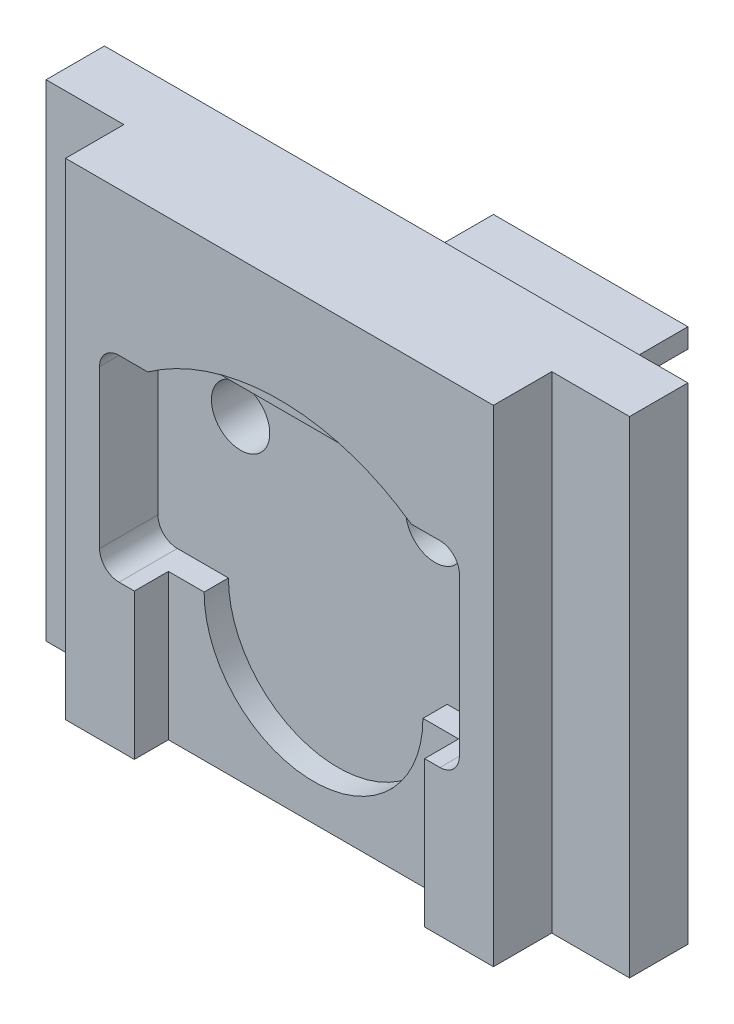
SolidWorks part; units mm, degrees
material "45"
ref_plane "前视基准面" through (0, 0, 0) normal (0, 0, 1) x (1, 0, 0)
ref_plane "上视基准面" through (0, 0, 0) normal (0, 1, 0) x (1, 0, 0)
ref_plane "右视基准面" through (0, 0, 0) normal (1, 0, 0) x (0, 0, -1)
sketch "草图1" plane through (0, 0, 0) normal (0, 0, 1) x (1, 0, 0)
  line L1 (30, -25) -> (-30, -25)
  line L2 (30, -25) -> (30, 25)
  line L3 (30, 25) -> (-30, 25)
  line L4 (-30, -25) -> (-30, 25)
  line L5 (30, -25) -> (-30, 25) construction
  line L6 (30, 25) -> (-30, -25) construction
  point P0 (0, 0)
  dimension "D1" = 60
  dimension "D2" = 50
extrude "凸台-拉伸1" add sketch "草图1" along normal blind 12
sketch "草图2" plane through (0, 0, 0) normal (0, 0, -1) x (-1, 0, 0)
  line L1 (10, -10) -> (-10, -10)
  line L2 (10, -10) -> (10, 10)
  line L3 (10, 10) -> (-10, 10)
  line L4 (-10, -10) -> (-10, 10)
  line L5 (10, -10) -> (-10, 10) construction
  line L6 (10, 10) -> (-10, -10) construction
  point P0 (0, 0)
  dimension "D1" = 20
  dimension "D2" = 20
extrude "凸台-拉伸2" add sketch "草图2" along normal blind 20
sketch "草图3" plane through (0, 0, 12) normal (0, 0, 1) x (1, 0, 0)
  line L0 (0, -25) -> (0, -10) construction
  line L1 (-30, -25) -> (30, -25) construction
  circle A0 centre (0, -10) radius 10.5
  dimension "D1" = 21
  dimension "D2" = 15
extrude "切除-拉伸1" cut sketch "草图3" against normal blind 6
sketch "草图5" plane through (0, 0, 12) normal (0, 0, 1) x (1, 0, 0)
  line L8 (-18.5, 4.9642) -> (-18.5, -1.5)
  line L9 (-17, -3) -> (-12.8452, -3)
  line L10 (12.8452, -3) -> (17, -3)
  line L11 (18.5, -1.5) -> (18.5, 4.9642)
  line L12 (-18.5, 4.9642) -> (-18.5, -1.5)
  line L13 (-17, -3) -> (-12.8452, -3)
  line L14 (12.8452, -3) -> (17, -3)
  line L15 (18.5, -1.5) -> (18.5, 4.9642)
  arc A16 (18.5, 4.9642) -> (18.1591, 5.9163) centre (17, 4.9642) ccw
  arc A17 (18.1591, 5.9163) -> (-18.1591, 5.9163) centre (0, -9) ccw
  arc A18 (-18.1591, 5.9163) -> (-18.5, 4.9642) centre (-17, 4.9642) ccw
  arc A19 (-18.5, -1.5) -> (-17, -3) centre (-17, -1.5) ccw
  arc A20 (-12.8452, -3) -> (-11.8311, -2.6053) centre (-12.8452, -1.5) ccw
  arc A21 (11.8311, -2.6053) -> (-11.8311, -2.6053) centre (0, -15.5) ccw
  arc A22 (11.8311, -2.6053) -> (12.8452, -3) centre (12.8452, -1.5) ccw
  arc A23 (17, -3) -> (18.5, -1.5) centre (17, -1.5) ccw
  arc A24 (18.5, 4.9642) -> (18.1591, 5.9163) centre (17, 4.9642) ccw
  arc A25 (18.1591, 5.9163) -> (-18.1591, 5.9163) centre (0, -9) ccw
  arc A26 (-18.1591, 5.9163) -> (-18.5, 4.9642) centre (-17, 4.9642) ccw
  arc A27 (-18.5, -1.5) -> (-17, -3) centre (-17, -1.5) ccw
  arc A28 (-12.8452, -3) -> (-11.8311, -2.6053) centre (-12.8452, -1.5) ccw
  arc A29 (11.8311, -2.6053) -> (-11.8311, -2.6053) centre (0, -15.5) ccw
  arc A30 (11.8311, -2.6053) -> (12.8452, -3) centre (12.8452, -1.5) ccw
  arc A31 (17, -3) -> (18.5, -1.5) centre (17, -1.5) ccw
  dimension "D1" = 0.5
extrude "切除-拉伸2" cut sketch "草图5" against normal blind 3.5
sketch "草图6" plane through (0, 0, 12) normal (0, 0, 1) x (1, 0, 0)
  line L0 (-17, -3) -> (-12.8452, -3) construction
  line L1 (-14.9226, -3) -> (14.9226, -3)
  line L2 (-14.9226, -3) -> (-14.9226, -25)
  line L3 (-14.9226, -25) -> (14.9226, -25)
  line L4 (14.9226, -3) -> (14.9226, -25)
  line L5 (-30, -25) -> (30, -25) construction
  line L6 (12.8452, -3) -> (17, -3) construction
  line L8 (13.3893, -8.4704) -> (-13.3893, -8.4704)
  line L9 (13.3893, -8.4704) -> (13.3893, 2.4704)
  line L10 (13.3893, 2.4704) -> (-13.3893, 2.4704)
  line L11 (-13.3893, -8.4704) -> (-13.3893, 2.4704)
  line L12 (13.3893, -8.4704) -> (-13.3893, 2.4704) construction
  line L13 (13.3893, 2.4704) -> (-13.3893, -8.4704) construction
  point P11 (0, -3)
  line M4 (17, -3) -> (12.8452, -3)
  arc M5 (12.8452, -3) -> (11.8311, -2.6053) centre (12.8452, -1.5) cw
  arc M6 (11.8311, -2.6053) -> (-11.8311, -2.6053) centre (0, -15.5) ccw
  arc M7 (-11.8311, -2.6053) -> (-12.8452, -3) centre (-12.8452, -1.5) cw
  line M8 (-12.8452, -3) -> (-17, -3)
  circle M13 centre (0, -10) radius 10.5
  line M15 (-30, -25) -> (30, -25)
extrude "切除-拉伸3" cut sketch "草图6" against normal blind 3.5 contours L8 L11 L1 L2 L4 L9 M15 M4 M13 | L8 L1 M13 | L1 M13 | L1 M7 M13 M5 M6 | L11 L8 L1 M13 M8 | L8 L9 L1 M13
sketch "草图7" plane through (0, 0, 8.5) normal (0, 0, 1) x (1, 0, 0)
  line L24 (-18.5, 0.05) -> (-18.5, 0)
  line L25 (-17, -1.5) -> (-12.3718, -1.5)
  line L26 (12.3718, -1.5) -> (17, -1.5)
  line L27 (18.5, 0) -> (18.5, 0.05)
  line L28 (3.937, 10.2) -> (-3.937, 10.2)
  line L29 (-18.5, 0.05) -> (-18.5, 0)
  line L30 (-17, -1.5) -> (-12.3718, -1.5)
  line L31 (12.3718, -1.5) -> (17, -1.5)
  line L32 (18.5, 0) -> (18.5, 0.05)
  line L33 (3.937, 10.2) -> (-3.937, 10.2)
  arc A36 (-5.7523, 9.8918) -> (-17.8817, 1.696) centre (3.72, -17.2) ccw
  arc A37 (-17.8817, 1.696) -> (-18.5, 0.05) centre (-16, 0.05) ccw
  arc A38 (-18.5, 0) -> (-17, -1.5) centre (-17, 0) ccw
  arc A39 (-10.1224, -5.0909) -> (-12.3718, -1.5) centre (-12.3718, -4) ccw
  arc A40 (-10.1224, -5.0909) -> (10.1224, -5.0909) centre (0, -10) ccw
  arc A41 (12.3718, -1.5) -> (10.1224, -5.0909) centre (12.3718, -4) ccw
  arc A42 (17, -1.5) -> (18.5, 0) centre (17, 0) ccw
  arc A43 (18.5, 0.05) -> (17.8817, 1.696) centre (16, 0.05) ccw
  arc A44 (17.8817, 1.696) -> (5.7523, 9.8918) centre (-3.72, -17.2) ccw
  arc A45 (5.7523, 9.8918) -> (3.937, 10.2) centre (3.937, 4.7) ccw
  arc A46 (-3.937, 10.2) -> (-5.7523, 9.8918) centre (-3.937, 4.7) ccw
  arc A47 (-5.7523, 9.8918) -> (-17.8817, 1.696) centre (3.72, -17.2) ccw
  arc A48 (-17.8817, 1.696) -> (-18.5, 0.05) centre (-16, 0.05) ccw
  arc A49 (-18.5, 0) -> (-17, -1.5) centre (-17, 0) ccw
  arc A50 (-10.1224, -5.0909) -> (-12.3718, -1.5) centre (-12.3718, -4) ccw
  arc A51 (-10.1224, -5.0909) -> (10.1224, -5.0909) centre (0, -10) ccw
  arc A52 (12.3718, -1.5) -> (10.1224, -5.0909) centre (12.3718, -4) ccw
  arc A53 (17, -1.5) -> (18.5, 0) centre (17, 0) ccw
  arc A54 (18.5, 0.05) -> (17.8817, 1.696) centre (16, 0.05) ccw
  arc A55 (17.8817, 1.696) -> (5.7523, 9.8918) centre (-3.72, -17.2) ccw
  arc A56 (5.7523, 9.8918) -> (3.937, 10.2) centre (3.937, 4.7) ccw
  arc A57 (-3.937, 10.2) -> (-5.7523, 9.8918) centre (-3.937, 4.7) ccw
  dimension "D1" = 0.5
extrude "切除-拉伸4" cut sketch "草图7" against normal blind 2.5
sketch "草图8" plane through (0, 0, 6) normal (0, 0, 1) x (1, 0, 0)
  circle A0 centre (-10, 5) radius 3
  circle A1 centre (10, 5) radius 3
  dimension "D1" = 6
extrude "切除-拉伸5" cut sketch "草图8" against normal up to next and the other way through all
sketch "草图9" plane through (0, 0, 12) normal (0, 0, 1) x (1, 0, 0)
  line L0 (-30, -25) -> (-14.9226, -25) construction
  line L1 (-30, 25) -> (-22, 25)
  line L2 (-30, 25) -> (-30, -25)
  line L3 (-30, -25) -> (-22, -25)
  line L4 (-22, 25) -> (-22, -25)
  line L5 (14.9226, -25) -> (30, -25) construction
  line L6 (30, -25) -> (22, -25)
  line L7 (30, -25) -> (30, 25)
  line L8 (30, 25) -> (22, 25)
  line L9 (22, -25) -> (22, 25)
  line L10 (30, 25) -> (-30, 25) construction
  dimension "D1" = 8
extrude "切除-拉伸6" cut sketch "草图9" against normal blind 6
sketch "草图10" plane through (0, 0, 8.5) normal (0, 0, 1) x (1, 0, 0)
  line L0 (0, -10) -> (-11.25, -10) construction
  line L1 (3.937, 10.2) -> (-3.937, 10.2) construction
  line L2 (-3.937, 10.2) -> (-18.5, 10.2)
  line L3 (-3.937, 10.2) -> (-3.937, -10)
  line L4 (-3.937, -10) -> (-18.5, -10)
  line L5 (-18.5, 10.2) -> (-18.5, -10)
  arc A0 (-10.1224, -5.0909) -> (10.1224, -5.0909) centre (0, -10) ccw construction
  arc A1 (-10.1224, -5.0909) -> (10.1224, -5.0909) centre (0, -10) ccw construction
  arc A2 (-3.937, 10.2) -> (-5.7523, 9.8918) centre (-3.937, 4.7) ccw construction
  arc A3 (-18.5, 0) -> (-17, -1.5) centre (-17, 0) ccw construction
extrude "切除-拉伸7" cut sketch "草图10" against normal up to surface (2.5 mm away) and the other way blind 10 up to face at (0, 1.5983, 6)
mirror "镜向2" about plane through (0, 0, 0) normal (1, 0, 0) of "切除-拉伸7"
fillet "圆角1" radius 2 4 edges at (18.5, -10, 9) (18.5, 10.2, 9) (-18.5, -10, 9) (-18.5, 10.2, 9)
